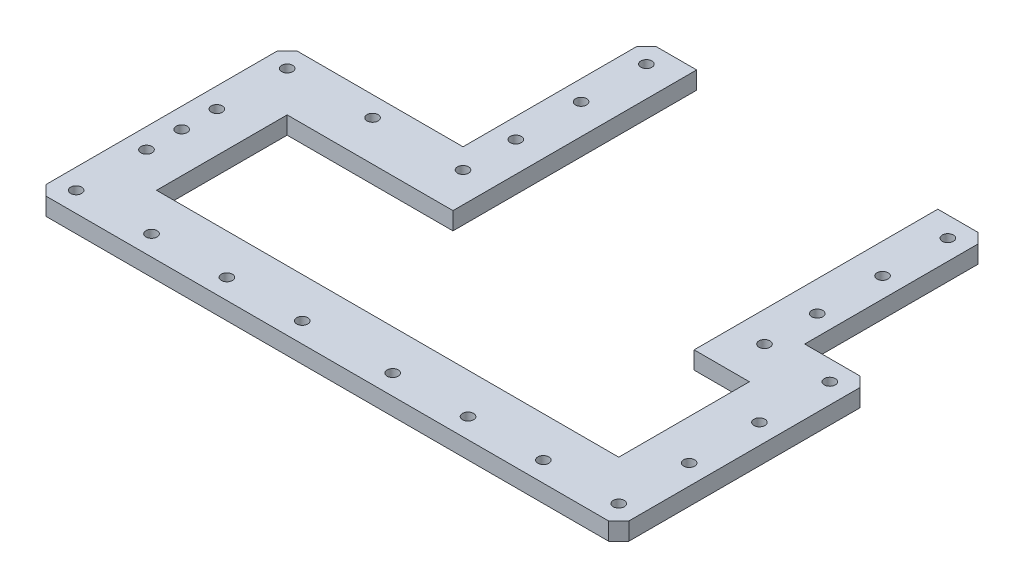
from build123d import *

# Parameters (mm, degrees)
BOSS_EXTRUDE1_DEPTH     = 35
CUT_EXTRUDE1_DEPTH      = 1448.428754723
CUT_EXTRUDE1_DEPTH_BACK = 1448.428754723
CHAMFER2_SIZE           = 20
CUT_EXTRUDE2_DEPTH      = 1448.428754723
CUT_EXTRUDE2_DEPTH_BACK = 1448.428754723
SKETCH5_R               = 11


with BuildPart() as part:
    # Sketch1 → Boss-Extrude1 (new body)
    with BuildSketch(Plane(origin=(0, 0, 0), x_dir=(1, 0, 0), z_dir=(0, 1, 0))):
        Polygon((-1160, 500), (-810, 500), (-810, 865), (-710, 865), (-710, 745), (-230, 745), (-230, 865), (-130, 865), (-130, 500), (0, 500), (0, 0), (-1160, 0), align=None)
    extrude(amount=BOSS_EXTRUDE1_DEPTH)

    # Sketch4 → Cut-Extrude1 (cut, two sides: drawn at the far end of the back side and taken through both)
    with BuildSketch(Plane(origin=(0, 35, 0), x_dir=(1, 0, 0), z_dir=(0, 1, 0)).offset(-CUT_EXTRUDE1_DEPTH_BACK)):
        Polygon((-230, 745), (-710, 745), (-710, 380), (-1040, 380), (-1040, 120), (-120, 120), (-120, 380), (-230, 380), align=None)
    extrude(amount=CUT_EXTRUDE1_DEPTH + CUT_EXTRUDE1_DEPTH_BACK, mode=Mode.SUBTRACT)

    # Chamfer2
    chamfer2_edges = [part.edges().sort_by_distance(p)[0] for p in [
        (0, 17.5, 0),
        (-1160, 17.5, 0),
        (-1160, 17.5, -500),
        (-810, 17.5, -865),
        (-130, 17.5, -865),
        (0, 17.5, -500),
    ]]
    chamfer(chamfer2_edges, length=CHAMFER2_SIZE)

    # Sketch5 → Cut-Extrude2 (cut, two sides: drawn at the far end of the back side and taken through both)
    with BuildSketch(Plane(origin=(0, 35, 0), x_dir=(1, 0, 0), z_dir=(0, 1, 0)).offset(-CUT_EXTRUDE2_DEPTH_BACK)):
        with Locations(Location((-1120, 40, 0), (0, 0, 270))):
            Circle(SKETCH5_R)
        with Locations(Location((-970, 40, 0), (0, 0, 270))):
            Circle(SKETCH5_R)
        with Locations(Location((-820, 40, 0), (0, 0, 270))):
            Circle(SKETCH5_R)
        with Locations(Location((-670, 40, 0), (0, 0, 270))):
            Circle(SKETCH5_R)
        with Locations(Location((-490, 40, 0), (0, 0, 270))):
            Circle(SKETCH5_R)
        with Locations(Location((-340, 40, 0), (0, 0, 270))):
            Circle(SKETCH5_R)
        with Locations(Location((-190, 40, 0), (0, 0, 270))):
            Circle(SKETCH5_R)
        with Locations(Location((-40, 40, 0), (0, 0, 270))):
            Circle(SKETCH5_R)
        with Locations(Location((-770, 825, 0), (0, 0, 270))):
            Circle(SKETCH5_R)
        with Locations(Location((-770, 695, 0), (0, 0, 270))):
            Circle(SKETCH5_R)
        with Locations(Location((-770, 565, 0), (0, 0, 270))):
            Circle(SKETCH5_R)
        with Locations(Location((-770, 460, 0), (0, 0, 270))):
            Circle(SKETCH5_R)
        with Locations(Location((-1120, 180, 0), (0, 0, 270))):
            Circle(SKETCH5_R)
        with Locations(Location((-1120, 250, 0), (0, 0, 270))):
            Circle(SKETCH5_R)
        with Locations(Location((-1120, 320, 0), (0, 0, 270))):
            Circle(SKETCH5_R)
        with Locations(Location((-1120, 460, 0), (0, 0, 270))):
            Circle(SKETCH5_R)
        with Locations(Location((-950, 460, 0), (0, 0, 270))):
            Circle(SKETCH5_R)
        with Locations(Location((-170, 460, 0), (0, 0, 90))):
            Circle(SKETCH5_R)
        with Locations(Location((-170, 565, 0), (0, 0, 90))):
            Circle(SKETCH5_R)
        with Locations(Location((-170, 695, 0), (0, 0, 90))):
            Circle(SKETCH5_R)
        with Locations(Location((-170, 825, 0), (0, 0, 90))):
            Circle(SKETCH5_R)
        with Locations(Location((-40, 460, 0), (0, 0, 270))):
            Circle(SKETCH5_R)
        with Locations(Location((-40, 320, 0), (0, 0, 270))):
            Circle(SKETCH5_R)
        with Locations(Location((-40, 180, 0), (0, 0, 270))):
            Circle(SKETCH5_R)
    extrude(amount=CUT_EXTRUDE2_DEPTH + CUT_EXTRUDE2_DEPTH_BACK, mode=Mode.SUBTRACT)


solid = part.part
